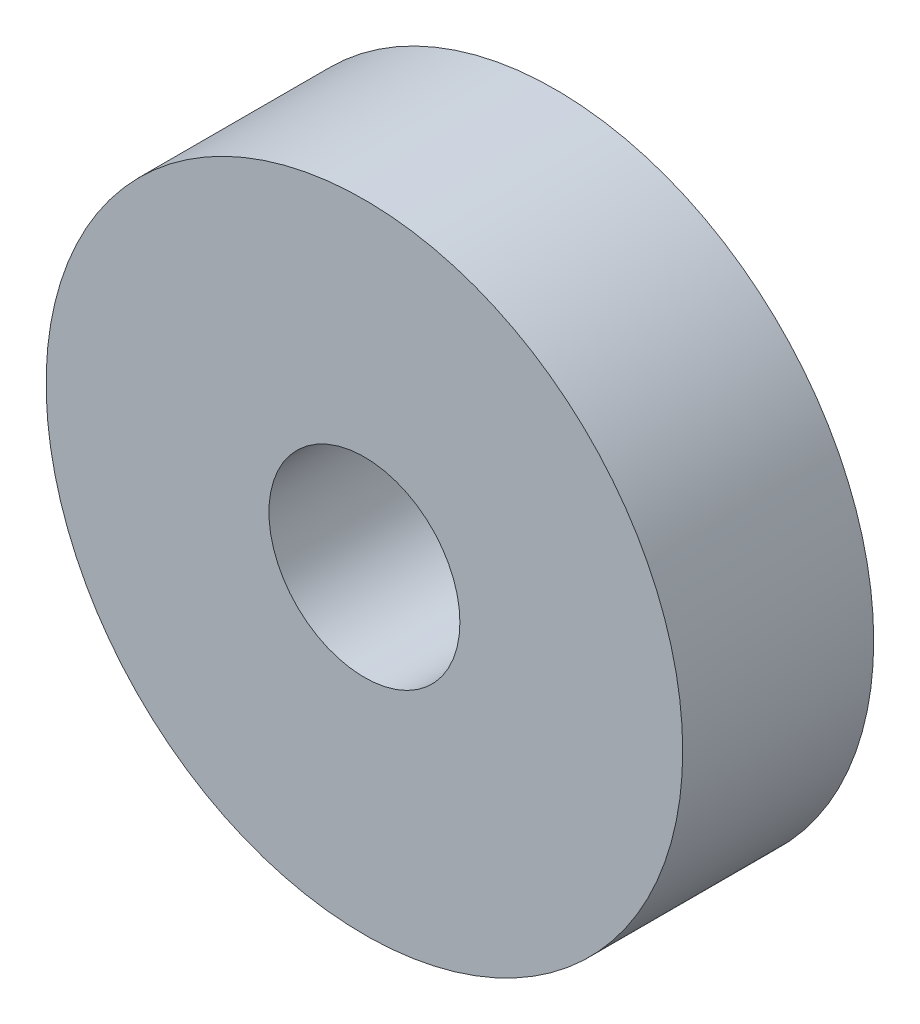
SolidWorks part; units mm, degrees
ref_plane "Front Plane" through (0, 0, 0) normal (0, 0, 1) x (1, 0, 0)
ref_plane "Top Plane" through (0, 0, 0) normal (0, 1, 0) x (1, 0, 0)
ref_plane "Right Plane" through (0, 0, 0) normal (1, 0, 0) x (0, 0, -1)
other "Configuration Table"
sketch "Sketch1" plane through (0, 0, 0) normal (0, 0, 1) x (1, 0, 0)
  circle A0 centre (0, 0) radius 10
  circle A1 centre (0, 0) radius 3
  dimension "D1" = 20
  dimension "D2" = 6
extrude "Boss-Extrude1" add sketch "Sketch1" along normal blind 6
